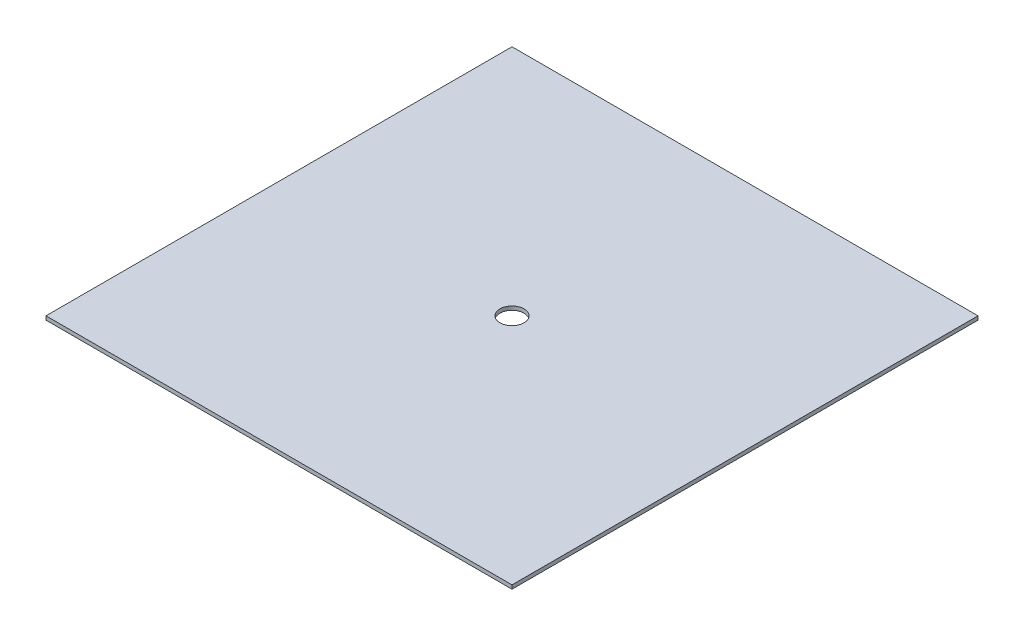
SolidWorks part; units mm, degrees
ref_plane "Front Plane" through (0, 0, 0) normal (0, 0, 1) x (1, 0, 0)
ref_plane "Top Plane" through (0, 0, 0) normal (0, 1, 0) x (1, 0, 0)
ref_plane "Right Plane" through (0, 0, 0) normal (1, 0, 0) x (0, 0, -1)
sketch "Sketch1" plane through (0, 0, 0) normal (0, 1, 0) x (1, 0, 0)
  line L1 (-49.2, -49.2) -> (49.2, -49.2)
  line L2 (-49.2, -49.2) -> (-49.2, 49.2)
  line L3 (-49.2, 49.2) -> (49.2, 49.2)
  line L4 (49.2, -49.2) -> (49.2, 49.2)
  line L5 (-49.2, -49.2) -> (49.2, 49.2) construction
  line L6 (-49.2, 49.2) -> (49.2, -49.2) construction
  circle A0 centre (0, 0) radius 2.55
  point P0 (0, 0)
  dimension "D2" = 5.1
  dimension "D1" = 98.4
extrude "Boss-Extrude1" add sketch "Sketch1" along normal blind 0.8
